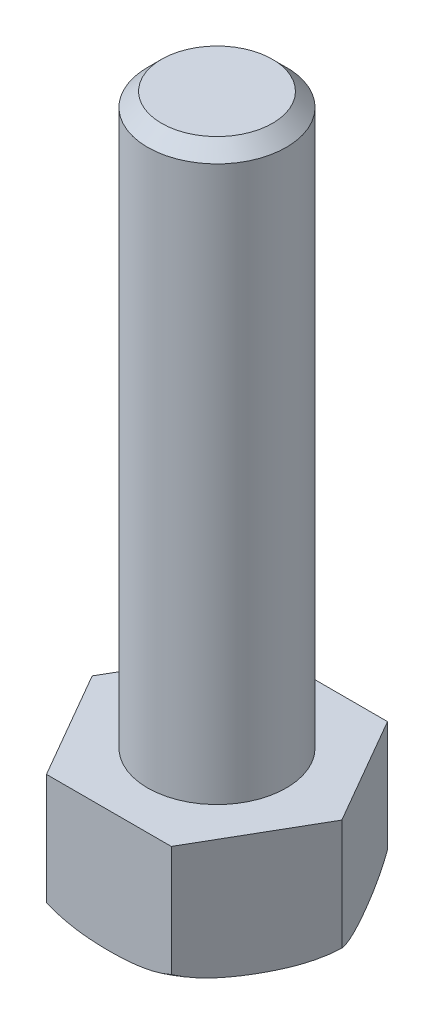
SolidWorks part; units mm, degrees
ref_plane "Front" through (0, 0, 0) normal (0, 0, 1) x (1, 0, 0)
ref_plane "Top" through (0, 0, 0) normal (0, 1, 0) x (1, 0, 0)
ref_plane "Right" through (0, 0, 0) normal (1, 0, 0) x (0, 0, -1)
sketch "Sketch1" plane through (0, 0, 0) normal (0, 0, 1) x (1, 0, 0)
  line L0 (0, 0) -> (9, 0)
  line L1 (9, 0) -> (9, 9)
  line L2 (9, 9) -> (5, 9)
  line L3 (5, 9) -> (5, 49)
  line L4 (5, 49) -> (4, 50)
  line L7 (4, 50) -> (0, 50)
  line L8 (0, 50) -> (0, 0)
  point P3 (5, 50)
  dimension "D1" = 9
  dimension "D2" = 9
  dimension "D3" = 50
revolve "Revolve1" add sketch "Sketch1" angle 360 about L8
sketch "Sketch2" plane through (0, 0, 0) normal (0, -1, 0) x (1, 0, 0)
  line L1 (9, 0) -> (4.5, 7.7942)
  line L2 (4.5, 7.7942) -> (-4.5, 7.7942)
  line L3 (-4.5, 7.7942) -> (-9, 0)
  line L4 (-9, 0) -> (-4.5, -7.7942)
  line L5 (-4.5, -7.7942) -> (4.5, -7.7942)
  line L6 (4.5, -7.7942) -> (9, 0)
  circle A0 centre (0, 0) radius 7.7942 construction
extrude "Cut-Extrude2" cut sketch "Sketch2" against normal blind 10 flip side to cut
sketch "Sketch5" plane through (0, 0, 0) normal (0, 0, 1) x (1, 0, 0)
  line L0 (-9, 0) -> (-9, 1)
  line L1 (-9, 0) -> (-7, 0)
  line L2 (0, 0) -> (0, 4.9597) construction
  arc A0 (-9, 1) -> (-7, 0) centre (-6.2824, 3.9351) ccw
  dimension "D3" = 4
  dimension "D1" = 1
  dimension "D2" = 2
revolve "Cut-Revolve2" cut sketch "Sketch5" angle 360 about L2
scale "Scale 1" bodies to scale 104 scale about centroid uniform scaling yes scale factor 1.875
